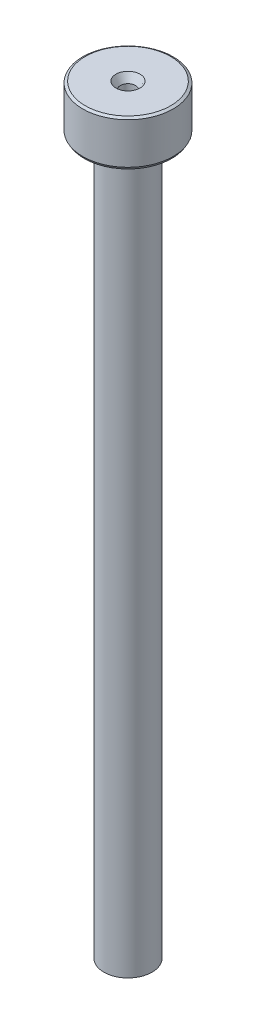
SolidWorks part; units mm, degrees
ref_plane "Front Plane" through (0, 0, 0) normal (0, 0, 1) x (1, 0, 0)
ref_plane "Top Plane" through (0, 0, 0) normal (0, 1, 0) x (1, 0, 0)
ref_plane "Right Plane" through (0, 0, 0) normal (1, 0, 0) x (0, 0, -1)
sketch "Sketch1" plane through (0, 0, 0) normal (0, 0, 1) x (1, 0, 0)
  line L1 (0, 252) -> (15, 252)
  line L2 (15, 252) -> (15, 237)
  line L4 (8, 233) -> (8, 0)
  line L5 (15, 237) -> (6, 237)
  line L6 (0, 252) -> (0, 0)
  line L7 (0, 0) -> (8, 0)
  line L9 (8, 233) -> (6, 233)
  line L10 (6, 237) -> (6, 233)
  dimension "D1" = 252
  dimension "D2" = 15
  dimension "D3" = 4
  dimension "D4" = 2
  dimension "D5" = 8
  dimension "D6" = 15
revolve "Revolve1" add sketch "Sketch1" angle 360 about L6
hole_wizard "Ø5.0mm Dowel Hole1" positions "Sketch2" profile "Sketch3" hole size "Ø5.0" standard "ISO"
sketch "Sketch2" plane through (0, 0, 0) normal (0, -1, 0) x (-1, 0, 0)
  point P0 (0, 0)
  point P4 (163.1935, -92.8029)
  point P6 (0, 0)
sketch "Sketch3" plane through (0, 0, 0) normal (1, 0, 0) x (0, 0, -1)
  line L0 (0, 0) -> (0, 6.5022)
  line L1 (0, 6.5022) -> (2.5, 5)
  line L2 (2.5, 5) -> (2.5, 0)
  line L5 (2.5, 0) -> (0, 0)
  line L10 (0, 6.5022) -> (-2.5, 5) construction
  line L11 (0, -6.35) -> (0, 107.95) construction
  dimension "Hole Dia." = 5
  dimension "Hole Depth" = 5
  dimension "Drill Angle" = 118
chamfer "Chamfer1" distance 1.5 angle 59 1 edges at (0, 0, -2.5)
chamfer "Chamfer2" distance 0.5 angle 59 3 edges at (-8, 233, 0) (-15, 237, 0) (-15, 252, 0)
hole_wizard "Ø5.0mm Dowel Hole2" positions "Sketch4" profile "Sketch5" hole size "Ø5.0" standard "ISO"
sketch "Sketch4" plane through (0, 252, 0) normal (0, 1, 0) x (1, 0, 0)
  point P0 (0, 0)
sketch "Sketch5" plane through (0, 252, 0) normal (1, 0, 0) x (0, 0, 1)
  line L0 (0, 0) -> (0, 6.5022)
  line L1 (0, 6.5022) -> (2.5, 5)
  line L2 (2.5, 5) -> (2.5, 0)
  line L5 (2.5, 0) -> (0, 0)
  line L10 (0, 6.5022) -> (-2.5, 5) construction
  line L11 (0, -6.35) -> (0, 107.95) construction
  dimension "Hole Dia." = 5
  dimension "Hole Depth" = 5
  dimension "Drill Angle" = 118
chamfer "Chamfer3" distance 1.5 angle 59 1 edges at (0, 252, 2.5)
